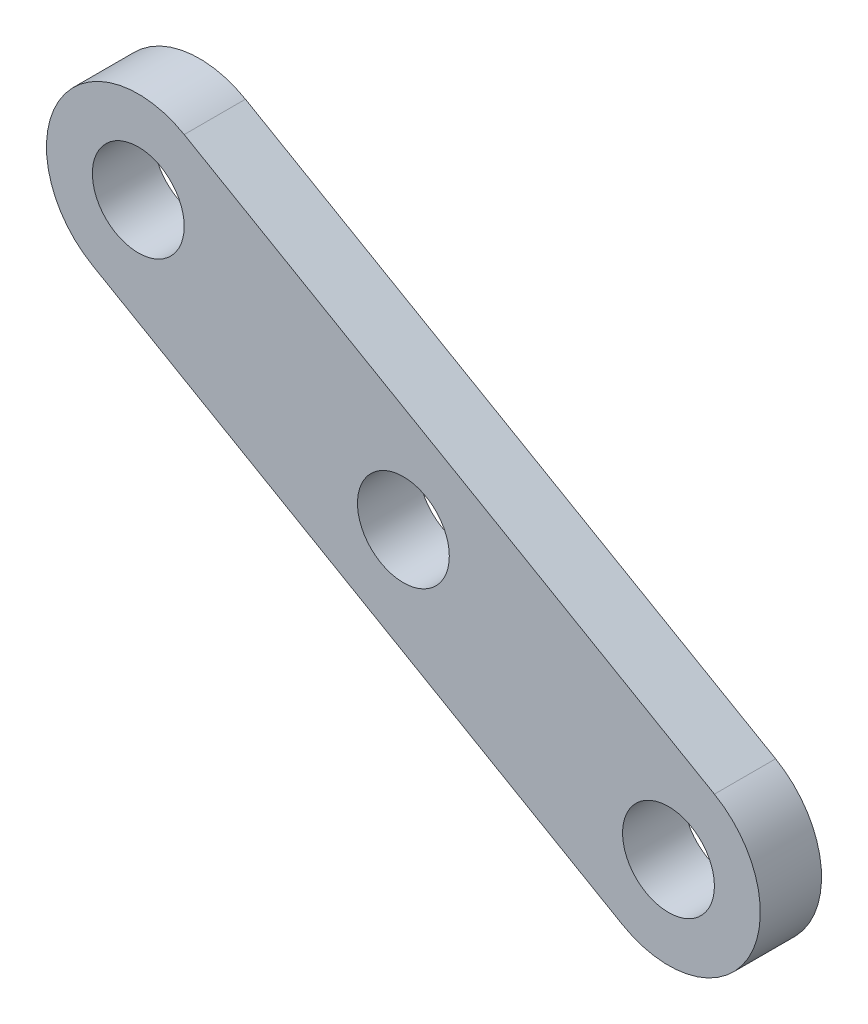
from build123d import *

# Parameters (mm, degrees)
SKETCH1_R           = 1.5
BOSS_EXTRUDE1_DEPTH = 2


with BuildPart() as part:
    # Sketch1 → Boss-Extrude1 (new body)
    with BuildSketch(Plane.XY):
        with BuildLine():
            Line((-10.160254038, 2.401923789), (7.160254038, -7.598076211))
            ThreePointArc((7.160254038, -7.598076211), (11.258330249, -6.5), (10.160254038, -2.401923789))
            Line((10.160254038, -2.401923789), (-7.160254038, 7.598076211))
            ThreePointArc((-7.160254038, 7.598076211), (-11.258330249, 6.5), (-10.160254038, 2.401923789))
        make_face()
        Circle(SKETCH1_R, mode=Mode.SUBTRACT)
        with Locations((8.660254038, -5)):
            Circle(SKETCH1_R, mode=Mode.SUBTRACT)
        with Locations((-8.660254038, 5)):
            Circle(SKETCH1_R, mode=Mode.SUBTRACT)
    extrude(amount=BOSS_EXTRUDE1_DEPTH)


solid = part.part
